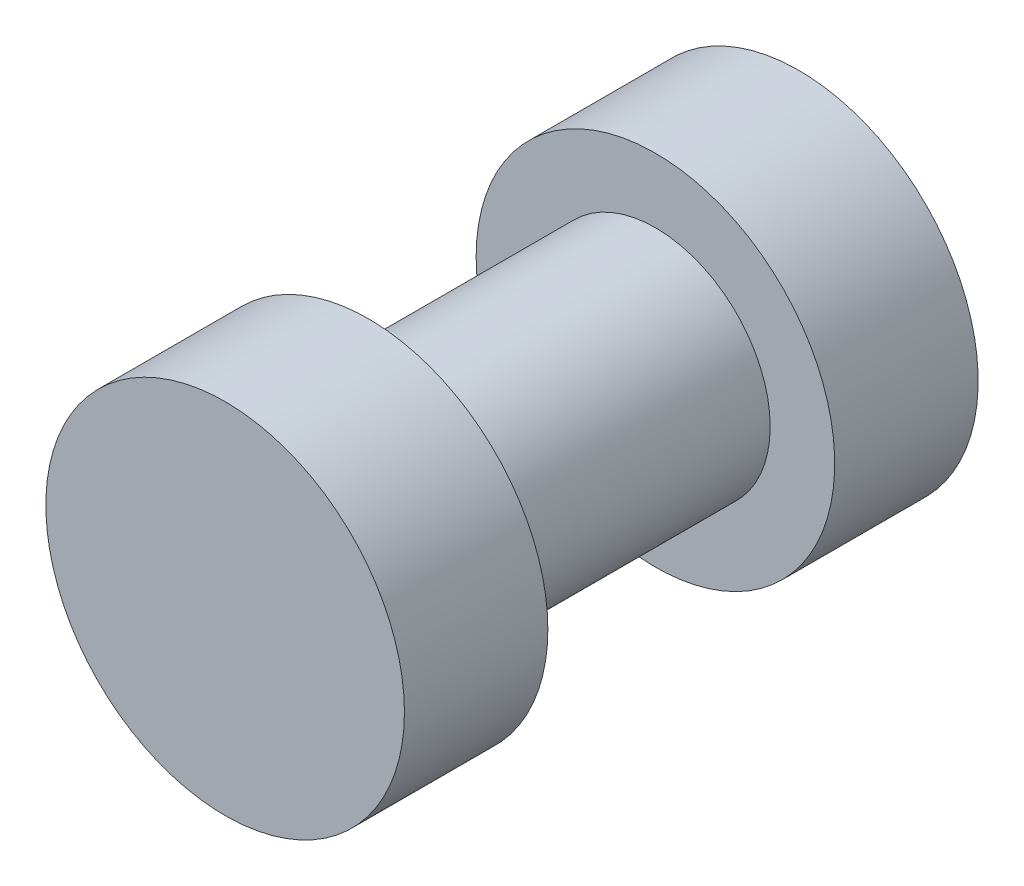
SolidWorks part; units mm, degrees
ref_plane "Front Plane" through (0, 0, 0) normal (0, 0, 1) x (1, 0, 0)
ref_plane "Top Plane" through (0, 0, 0) normal (0, 1, 0) x (1, 0, 0)
ref_plane "Right Plane" through (0, 0, 0) normal (1, 0, 0) x (0, 0, -1)
sketch "Sketch1" plane through (0, 0, 0) normal (0, 0, 1) x (1, 0, 0)
  circle A0 centre (0, 0) radius 8
  dimension "D1" = 16
extrude "Boss-Extrude1" add sketch "Sketch1" along normal blind 20
sketch "Sketch2" plane through (0, 0, 20) normal (0, 0, 1) x (1, 0, 0)
  circle A0 centre (0, 0) radius 12.5
  dimension "D1" = 25
extrude "Boss-Extrude2" add sketch "Sketch2" along normal blind 10
sketch "Sketch3" plane through (0, 0, 0) normal (0, 0, -1) x (-1, 0, 0)
  circle A0 centre (0, 0) radius 12.5
  dimension "D1" = 25
extrude "Boss-Extrude3" add sketch "Sketch3" along normal blind 10
